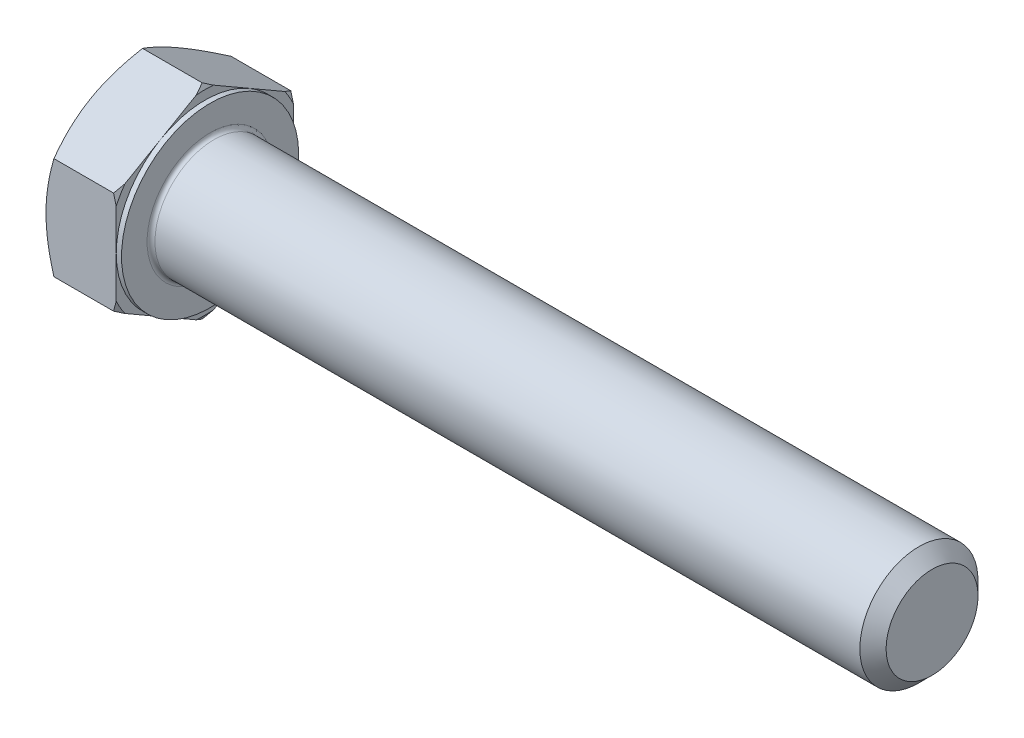
from build123d import *

# Parameters (mm, degrees)
EXTRUDE_371_DEPTH = 11.5
SKETCH_4_W        = 0.8
SKETCH_4_H        = 12.088457268
CHAMFER_2038_SIZE = 2
FILLET_2080_R     = 0.6


with BuildPart() as part:
    # 草图1 → Extrude 371 (new body)
    with BuildSketch(Plane(origin=(0, 0, 0), x_dir=(0, 0, -1), z_dir=(1, 0, 0))):
        Polygon((13.5, 7.794228634), (13.5, -7.794228634), (0, -15.588457268), (-13.5, -7.794228634), (-13.5, 7.794228634), (0, 15.588457268), align=None)
    extrude(amount=EXTRUDE_371_DEPTH)

    # 草图2 → 凸台-旋转1 (revolve)
    with BuildSketch(Plane.XY, mode=Mode.PRIVATE) as revolve_1_sk:
        Polygon((0, 0), (121.5, 0), (121.5, 6.835), (121.5, 9), (27.8072, 9), (0, 9), align=None)
    revolve(revolve_1_sk.sketch.rotate(Axis((0, 0, 0), (1, 0, 0)), 90), axis=Axis((0, 0, 0), (1, 0, 0)))

    # 草图3 → 切除-旋转1 (revolve, cut)
    with BuildSketch(Plane.XY):
        Polygon((0, 13.5), (4.092522712, 20.588457268), (4.092522712, 25.588457268), (-10, 25.588457268), (-10, 13.5), align=None)
    revolve(axis=Axis((0, 0, 0), (1, 0, 0)), mode=Mode.SUBTRACT)

    # 草图5 → 切除-旋转2 (revolve, cut)
    with BuildSketch(Plane.XY):
        Polygon((11.5, 13.5), (7.407477288, 20.588457268), (7.407477288, 25.588457268), (17.407477288, 25.588457268), (17.407477288, 13.5), align=None)
    revolve(axis=Axis((0, 0, 0), (1, 0, 0)), mode=Mode.SUBTRACT)

    # 草图4 → 切除-旋转3 (revolve, cut)
    with BuildSketch(Plane.XY, mode=Mode.PRIVATE) as cut_revolve_3_sk:
        with Locations((11.1, 19.544228634)):
            Rectangle(SKETCH_4_W, SKETCH_4_H)
    revolve(cut_revolve_3_sk.sketch.rotate(Axis((0, 0, 0), (1, 0, 0)), 270), axis=Axis((0, 0, 0), (1, 0, 0)), mode=Mode.SUBTRACT)

    # Chamfer 2038
    chamfer_2038_edges = [part.edges().sort_by_distance(p)[0] for p in [
        (121.5, 0, -9),
    ]]
    chamfer(chamfer_2038_edges, length=CHAMFER_2038_SIZE)

    # Fillet 2080
    fillet_2080_edges = [part.edges().sort_by_distance(p)[0] for p in [
        (11.5, 0, -9),
    ]]
    fillet(fillet_2080_edges, radius=FILLET_2080_R)


solid = part.part
